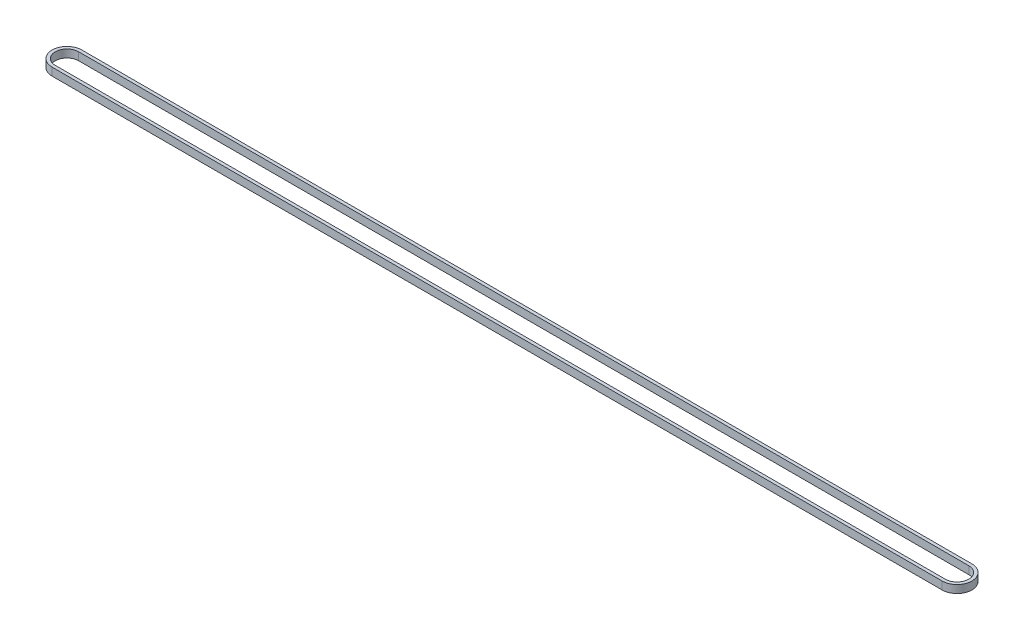
from build123d import *

# Parameters (mm, degrees)
BOSS_EXTRUDE1_DEPTH = 5


with BuildPart() as part:
    # Sketch1 → Boss-Extrude1 (new body)
    with BuildSketch(Plane(origin=(0, 0, 0), x_dir=(1, 0, 0), z_dir=(0, 1, 0))):
        with BuildLine():
            Line((284.5, -9.5), (-284.5, -9.5))
            ThreePointArc((-284.5, -9.5), (-294, 0), (-284.5, 9.5))
            Line((-284.5, 9.5), (284.5, 9.5))
            ThreePointArc((284.5, 9.5), (294, 0), (284.5, -9.5))
        make_face()
        with BuildLine():
            Line((284.5, -7.5), (-284.5, -7.5))
            ThreePointArc((-284.5, -7.5), (-292, 0), (-284.5, 7.5))
            Line((-284.5, 7.5), (284.5, 7.5))
            ThreePointArc((284.5, 7.5), (292, 0), (284.5, -7.5))
        make_face(mode=Mode.SUBTRACT)
    extrude(amount=BOSS_EXTRUDE1_DEPTH)


solid = part.part
